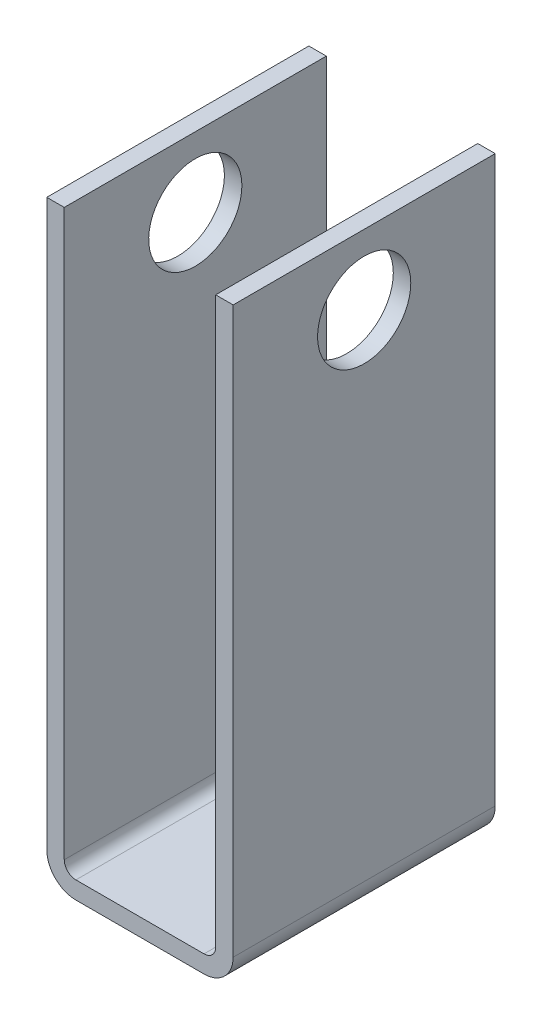
SolidWorks part; units mm, degrees
ref_plane "Front Plane" through (0, 0, 0) normal (0, 0, 1) x (1, 0, 0)
ref_plane "Top Plane" through (0, 0, 0) normal (0, 1, 0) x (1, 0, 0)
ref_plane "Right Plane" through (0, 0, 0) normal (1, 0, 0) x (0, 0, -1)
sketch "Sketch1" plane through (0, 0, 0) normal (0, 0, 1) x (1, 0, 0)
  line L0 (0, 0) -> (0, -97)
  line L1 (5, -102) -> (27, -102)
  line L2 (32, -97) -> (32, 0)
  line L3 (3, 0) -> (3, -97)
  line L4 (5, -99) -> (27, -99)
  line L5 (29, -97) -> (29, 0)
  line L6 (3, 0) -> (0, 0)
  line L7 (29, 0) -> (32, 0)
  arc A0 (27, -102) -> (32, -97) centre (27, -97) ccw
  arc A1 (0, -97) -> (5, -102) centre (5, -97) ccw
  arc A2 (3, -97) -> (5, -99) centre (5, -97) ccw
  arc A3 (27, -99) -> (29, -97) centre (27, -97) ccw
  point P8 (32, -102)
  point P11 (0, -102)
  dimension "D3" = 5
  dimension "D1" = 32
  dimension "D2" = 102
  dimension "D4" = 3
extrude "Boss-Extrude1" add sketch "Sketch1" along normal blind 45
sketch "Sketch2" plane through (32, 0, 0) normal (1, 0, 0) x (0, 0, -1)
  line L0 (0, -97) -> (0, 0) construction
  line L1 (-45, 0) -> (0, 0) construction
  circle A0 centre (-22.5, -12) radius 8
  dimension "D1" = 16
  dimension "D2" = 22.5
  dimension "D3" = 12
extrude "Cut-Extrude1" cut sketch "Sketch2" against normal through all
